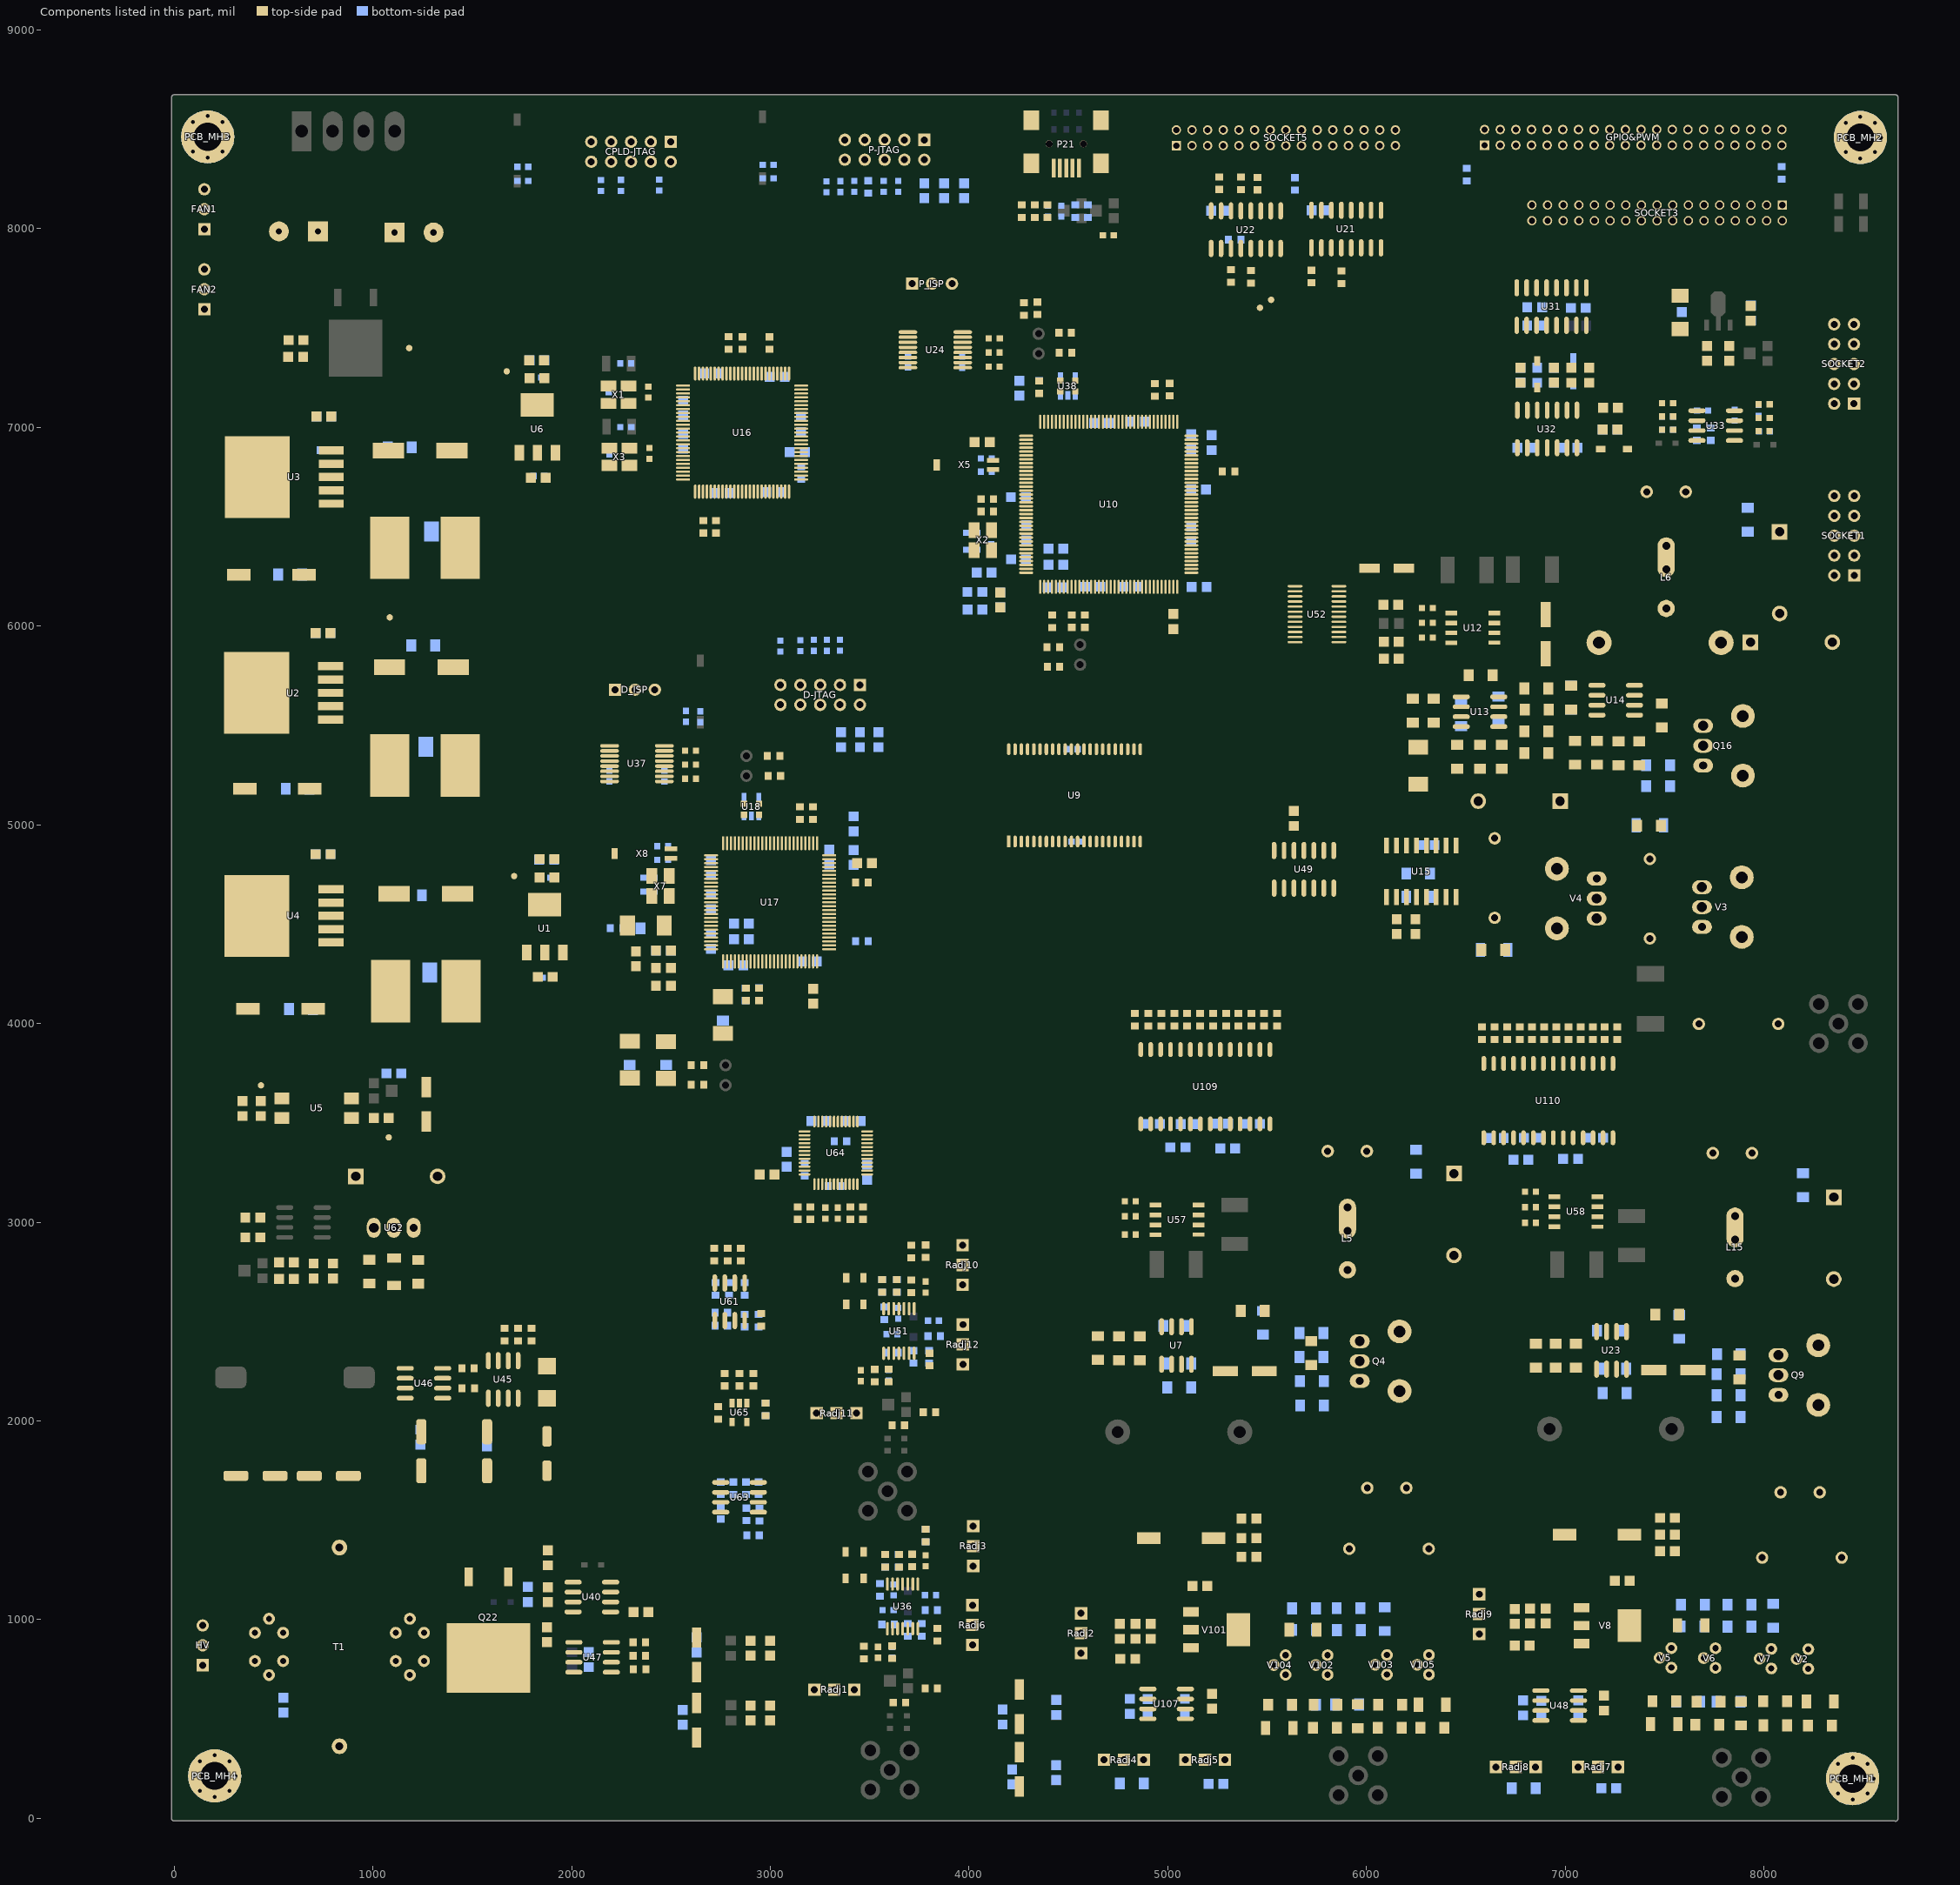
[diagram p0: the components of this part, seen from the top]
# Altium PCB MISC82309.PcbDoc (part 3 of 14)
Units mil, origin at the board's own origin, x right, y up, seen from the top; angles counter-clockwise.
Board outline 8687.03 x 8687.86 mil, 4 copper layers (Top Layer, GND, POWER, Bottom Layer); 747 components, 583 nets, 2530 pads, 1834 vias.

## Components (designator, comment, footprint, x,y, rotation, side; value= is the part's Value field where it differs from the comment) (continued)
R187 "200K" RES_0603 3470,835 r90 top
R188 "6.8K" RES_0603 3593,975 r0 bottom
R189 "6.8K" RES_0603 3646,1297 r90 bottom
R190 "18K" RES_0603 3577,1297 r270 bottom
R191 "27K" RES_0603 3577,1297 r90 top
R192 "15K" RES_0603 3552,1150 r90 bottom
R193 "3.9K" RES_0603 3647,1297 r90 top
R194 "1.5K" RES_0603 3713,1298 r270 top
R195 "27K" RES_0603 3782,1424 r270 bottom
R196 "30K" RES_0603 3782,1424 r270 top
R197 "15K" RES_0603 3761,948 r90 bottom
R198 "1K" RES_0603 3691,948 r270 bottom
R199 "100K" RES_0603 3841,924 r90 top
R200 "10K" RES_0603 3810,1048 r0 bottom
R201 "390R" R1206 5565,572 r180 top
R202 "2K2" R1206 5956,514 r270 top
R203 "100R" R1206 5791,456 r0 top
R204 "100R" R0805 3000,530 r90 top
R205 "100R" R0805 2999,856 r90 top
R206 "1K" R1206 2406,4479 r0 bottom
R207 "1K" R1206 2292,3851 r90 bottom
R208 "4.7K" R0603 4535,7208 r270 top
R209 "4.7K" R0603 4459,7208 r270 top
R212 "100R" R0805 6797,6898 r0 bottom
R213 "33R" RES_0603 1480,2165 r0 top
R214 "33R" RES_0603 1479,2265 r0 top
R215 "33R" RES_0805 1877,924 r270 top
R216 "150K" R0805 1881,1126 r270 top
R217 "100K" R0805 1880,1311 r90 top
R220 "1K" R0805 2349,1039 r0 top
R221 "1K8" R1206 6852,2329 r90 top
R222 "0R" R0805 2324,4326 r270 top
R225 "47R" R0805 2702,4414 r90 bottom
R226 "1K" RES_0603 4599,8088 r90 bottom
R227 "150K" R1206 7514,2535 r0 top
R232 "10K" R0603 2248,8218 r270 bottom
R234 "10K" R0603 2148,8217 r270 bottom
R235 "0R" R0805 2462,4190 r180 top
R236 "56K" R1206 7573,2474 r270 bottom
R269 "0R" R0805 4076,6268.51 r180 bottom
R270 "1K" RES_0603 4425,5795 r180 top
R271 "1K" RES_0603 4484,7476 r0 top
R272 "1K" RES_0603 2634,3691 r180 top
R273 "1K" RES_0603 3017,5347 r0 top
R274 "0R" RES_0603 4353,7202.5 r90 top
R275 "0R/NC" RES_0603 4353,7203 r270 bottom
R276 "47R" R0805 4249,6336 r0 bottom
R277 "0R" R0805 4030,6083 r180 bottom
R283 "4.7K" R0805 7713,7373 r270 top
R284 "560R" R0805 7825,7372 r90 top
R285 "100R" RES_0603 1731,2435 r270 top
R286 "10K" RES_0603 1799,2435 r90 top
R287 "10K" RES_0603 2342,751 r0 top
R288 "100R" RES_0603 2341,818 r180 top
R290 "50R" RES_0805 7066,556 r90 bottom
R291 "470R" RES_0805 7287,1195 r0 top
R292 "3K3" RES_0805 7194,580 r270 top
R293 "0R" RES_0805 550,570 r270 bottom
R294 "10K" R0603 2441,8219 r90 bottom
R295 "2K7" RES_0805 7514,1427 r0 top
R296 "2K7" RES_0805 7514,1512 r180 top
R297 "1K" R1206 8046,1019 r90 bottom
R298 "1K5" R1206 7721,588 r0 top
R299 "1K5" R1206 8056,589 r0 top
R300 "390R" R1206 7499,589 r180 top
R301 "390R" R1206 8282,467 r0 top
R302 "2K2" R1206 7884,528 r270 top
R303 "100R" R1206 7714,472 r0 top
R304 "100R" R1206 8057,468 r0 top
R305 "150K" R1206 7618,588 r180 bottom
R306 "1.8K" R1206 7822,588 r180 bottom
R307 "12K" R1206 7876,965 r180 bottom
R308 "12K" R1206 7876,1075 r0 bottom
R309 "12K" R1206 7643,1075 r0 bottom
R310 "12K" R1206 7640,966 r180 bottom
R312 "10K" R0603 4811.5,3030 r180 top
R313 "1M" R1206 8196,3186 r270 bottom
R314 "50R" RES_0805 6746,1017 r270 top
R315 "510R" RES_0805 6788,556 r90 bottom
R316 "50R" RES_0805 6901,1018 r90 top
R317 "20R" RES_0805 6823,1018 r270 top
R318 "2K" RES_0805 6777,3315 r0 bottom
R319 "1M" R1206 6952,2329 r90 top
R320 "2.7K" RES_0805 6879,555 r270 bottom
R321 "100R" RES_0805 6784,869 r0 top
R322 "10K" RES_0603 3595,2229 r90 top
R323 "200K" RES_0603 3526,2228 r90 top
R324 "6.8K" RES_0603 3611,2343 r0 bottom
R325 "6.8K" RES_0603 3637,2680 r90 bottom
R326 "18K" RES_0603 3563,2680 r270 bottom
R327 "27K" RES_0603 3563,2680 r90 top
R328 "15K" RES_0603 3574,2542 r90 bottom
R329 "3.9K" RES_0603 3636,2680 r90 top
R330 "1.5K" RES_0603 3709,2677 r270 top
R331 "27K" RES_0603 3710,2853 r270 top
R332 "30K" RES_0603 3782,2854 r270 top
R333 "15K" RES_0603 3721,2322 r90 bottom
R334 "1K" RES_0603 3800,2322 r270 bottom
R336 "10K" RES_0603 3825,2428 r0 bottom
R339 "100K" RES_0603 3802,2309 r90 top
R343 "10K" R0603 6825,2997 r180 top
R344 "10K" R0603 6825,3076 r180 top
R345 "0R" RES_0603 2663,6500 r270 top
R346 "0R" RES_0603 2727,6500 r270 top
R347 "0R" RES_0603 2996,7424 r90 top
R348 "0R/NC" RES_0603 4583,6025 r270 top
R349 "0R/NC" RES_0603 4517,6025 r270 top
R358 "0R" RES_0603 6504,8272 r270 bottom
R372 "330K" R0603 8001,7116 r0 top
R373 "1M" R0603 8001,7048 r0 top
R374 "330K" R0603 7973,7085 r90 bottom
R375 "0ohm" R0603 8000,6982 r180 top
R378 "4.7K" RES_0603 3810,655 r0 top
R379 "4.7K" RES_0603 3801,2045 r0 top
R386 "100R" R0805 5635,5032 r90 top
R391 "0R/NC" RES_0603 4092,6577 r180 top
R392 "0R" RES_0603 4092,6639.17 r180 top
R399 "100R" RES_0805 396,2924 r180 top
R404 "10K" RES_0603 8090,8281 r90 bottom
R405 "0R" RES_0603 5318,7762 r90 top
R406 "0R" RES_0603 3492,8210 r90 bottom
R407 "0R" RES_0603 5724,7759 r90 top
R408 "0R" RES_0603 5418,7758 r90 top
R409 "0R/NC" RES_0603 2861,7424 r90 top
R410 "0R/NC" RES_0603 2790,7425 r90 top
R411 "51R" RES_0603 2942,2505 r90 bottom
R412 "499R" RES_0603 2871,2505.51 r270 bottom
R413 "499R" RES_0603 2792,2664 r270 bottom
R414 "499R" RES_0603 2753,2480 r0 bottom
R415 "33R" RES_0603 3202,3046 r90 top
R416 "33R" RES_0603 3137,3046 r270 top
R417 "499R" RES_0603 2872,2664 r270 bottom
R418 "33R" RES_0603 3403,3046 r270 top
R419 "33R" RES_0603 3466,3046 r90 top
R455 "0R/NC" RES_0603 3156,6770 r270 bottom
R478 "0R/NC" RES_0603 2954,2509 r270 top
R479 "0R" RES_0603 2770,2208 r90 top
R491 "680R" R0805 7120,7262 r270 top
R493 "680R" R0805 7228,7098 r180 top
R495 "1K" R0805 6944,7262 r270 bottom
R496 "1K" R0805 7225,6989 r180 top
R508 "0R" RES_0603 5306,6778 r0 top
R509 "0R" RES_0603 5009,7190 r270 top
R511 "0R" RES_0603 4936,7188 r270 top
R513 "0R" RES_0603 3214,5059 r90 top
R514 "0R" RES_0603 3150,5059 r90 top
R515 "0R/NC" RES_0603 2877,4147 r270 top
R516 "0R/NC" RES_0603 2943,4147 r270 top
R517 "499R" RES_0603 2750,1538 r270 bottom
R518 "0R" RES_0603 3461,4709 r0 top
R519 "0R" RES_0603 3461,4414 r0 bottom
R521 "51R" RES_0603 2913,1425 r180 bottom
R522 "499R" RES_0603 2879,1530 r270 bottom
R523 "499R" RES_0603 2942,1661 r270 bottom
R524 "499R" RES_0603 2750.51,1661 r270 bottom
R525 "0R" RES_0603 5098,4019 r90 top
R526 "0R" RES_0603 5163,4019 r90 top
R527 "0R" RES_0603 5228,4019 r90 top
R528 "0R" RES_0603 5293,4019 r90 top
R529 "0R" RES_0603 5356,4019 r90 top
R530 "0R" RES_0603 5421,4019 r90 top
R531 "0R" RES_0603 5485,4019 r90 top
R532 "0R" RES_0603 5550,4019 r90 top
R533 "0R" RES_0603 6581,3951.5 r90 top
R534 "0R" RES_0603 6645,3951.5 r90 top
R535 "0R" RES_0603 6708,3951.5 r90 top
R536 "0R" RES_0603 6771,3951.5 r90 top
R537 "0R" RES_0603 6832,3951.5 r90 top
R538 "0R" RES_0603 6893,3951.5 r90 top
R539 "0R" RES_0603 6955,3951.5 r90 top
R540 "0R" RES_0603 7016,3951.5 r90 top
R541 "0R" RES_0603 7077,3951.5 r90 top
R542 "0R" RES_0603 7138,3951.5 r90 top
R543 "0R" RES_0603 7199,3951.5 r90 top
R544 "0R" RES_0603 7262,3951.5 r90 top
R545 "1M/NC" RES_0603 3650,583 r180 top
R546 "1M/NC" RES_0603 3644,1978 r180 top
R547 "0R" RES_0603 4835,4019 r90 top
R548 "0R" RES_0603 4902,4019 r90 top
R549 "0R" RES_0603 4968,4019 r90 top
R550 "0R" RES_0603 5034,4019 r90 top
R555 "0R/NC" RES_0603 767,6885 r0 bottom
R556 "0R" RES_0603 2227,4479 r180 bottom
R558 "0R" RES_0603 4418,6024 r270 top
R564 "0R/NC" RES_0603 2943,4148 r90 bottom
R565 "0R/NC" RES_0603 2876,4147 r90 bottom
R567 "0R/NC" RES_0603 4343,7599 r270 top
R569 "0R/NC" RES_0603 4276,7596 r270 top
R578 "0R/NC" RES_0603 2945,1529 r270 bottom
R587 "10K" R0603 3570,8213 r270 bottom
R588 "10K" R0603 3353,8212 r270 bottom
R589 "10K" R0603 3643,8213 r270 bottom
R590 "10K" R0603 3423,8213 r270 bottom
R591 "10K" R0603 3283,8211 r90 bottom
R592 "10K" R0603 3351,5904 r90 bottom
R593 "10K" R0603 3219,5903 r90 bottom
R594 "10K" R0603 3151,5902 r90 bottom
R595 "10K" R0603 3051,5899 r270 bottom
R596 "10K" R0603 3285,5903 r270 bottom
R598 "10K" RES_0603 2852,2838 r90 top
R599 "10K" RES_0603 2785,2838 r270 top
Radj1 "10K" Radj 3422,648 r180 top
Radj2 "10K" Radj 4564,832 r90 top
Radj3 "10K" Radj 4021,1470 r270 top
Radj4 "2K" Radj 4679,295 r0 top
Radj5 "5K" Radj 5088,295 r0 top
Radj6 "10K" Radj 4017,1073 r270 top
Radj7 "5K" Radj 7065,259 r0 top
Radj8 "2K" Radj 6651,259 r0 top
Radj9 "10K" Radj 6567,928 r90 top
Radj10 "10K" Radj 3967,2885 r270 top
Radj11 "10K" Radj 3433,2039 r180 top
Radj12 "10K" Radj 3969,2485 r270 top
SOCKET1 "IDC2X5-2_54" IDC2X5-2_54 8454,6255 r90 top
SOCKET2 "IDC2X5-2_54" IDC2X5-2_54 8453,7119 r90 top
SOCKET3 "HEAD2X17-2MM-A" IDC2X17-2.0mm-A 8092,8119 r180 top
SOCKET5 "HEAD2X15-2MM-A" IDC2X15-2.0mm-A 5043,8418 r0 top
T1 "Trans1" RM8 832,863 r180 top
TC2 "220uF/25V" E8X10,2 4904,1411 r0 top
TC3 "220uF/25V" E8X10,2 6997,1427 r0 top
TP1 "TP" TPOINT 1711,4742 r90 top
TP2 "TP" TPOINT 1085,6044 r90 top
TP3 "TP" TPOINT 1080,3427 r270 top
TP4 "TP" TPOINT 437,3689 r270 top
TP5 "TP" TPOINT 1183,7399 r90 top
TP6 "TP" TPOINT 1674,7282 r90 top
TP7 "TP" TPOINT 5520,7642 r90 top
TP8 "TP" TPOINT 5464,7602 r90 top
U1 "AMS1117-3.3V" SOT223 1775,4358 r90 top
U2 "LM2596S-12" TS5B_N 551,5664 r180 top
U3 "LM2596S-5.0" TS5B_N 554,6750 r180 top
U4 "LM2596S-12" TS5B_N 553,4542 r180 top
U5 "PC817" SOIC_4N 718,3574 r180 top
U6 "AMS1117-3.3V" SOT223 1738,6872 r90 top
U7 "UC3842D" SOIC-8 5044,2380 r270 top
U9 "IS61LV51216AL" TSOP44-IS61LV51216AL-10TLI 4200,4916 r90 top
U10 "STM32F407ZET6" LQFP144 4703,6613 r0 top
U12 "ISP742RI" P-DSO-8 6427,6066 r0 top
U13 "TL082ACD" SO8 6571,5569 r0 top
U14 "UC3842D" SOIC-8 7254,5627 r0 top
U15 "IR2113" SOIC-16 6276,4766 r90 top
U16 "EPM240GT100C5N" TQFP100_N 2858,6974 r270 top
U17 "STM32F407VGT6" LQFP100_N 2999,4610 r0 top
U18 "DS28CM00R-A00+T" U5+1_N 2905,5092 r90 bottom
U21 "MC3487D" 751B-03_N 5898,7998 r90 top
U22 "MC3486D" 751B-03_N 5393,7995 r90 top
U23 "UC3842D" SOIC-8 7233,2355 r270 top
U24 "SP3232EEA" SSOP16_M 3830,7390 r180 top
U31 "MC3486D" 751B-03 6931,7608 r270 top
U32 "M74HCT14M1R" SO14_N 6909,6992 r270 top
U33 "LM358D" SO8_N 7757,7009 r180 top
U36 "MC33074DTB" 948G-01_N 3666,1067 r90 top
U37 "SP3232EEA" SSOP16_M 2329,5308 r180 top
U38 "DS28CM00R-A00+T" U5+1_N 4497,7208 r90 bottom
U40 "LM358D" SO8_N 2102,1114 r0 top
U45 "IR2184S" SOIC_8N 1656,2209 r270 top
U46 "IRF7341" SOIC_8N 1257,2190 r180 top
U47 "MC33152D" 751-05_N 2106,811 r180 top
U48 "TLE2082AID" SOIC-8 6972,568 r180 top
U49 "M74HCT14M1R" SO14 5685,4776 r90 top
U51 "MC33074DTB" 948G-01_N 3647,2453 r90 top
U52 "SN74LVC4245PW" TSSOP-24 5751,6060 r180 top
U57 "ISP742RI" P-DSO-8 4939,3087 r0 top
U58 "ISP742RI" P-DSO-8 6946,3128 r0 top
U61 "ADC8138" SO8 2796,2600 r270 top
U62 "MC7815ACT" TO220 1105,2972 r90 top
U63 "ADC8138" SO8_N 2845,1616 r180 top
U64 "AD9288BST100" LQFP48A 3330,3349 r90 top
U65 "TPS60403" SOT23-5_M 2845,2042 r90 top
U107 "TLE2082AID" SOIC-8 4994,576 r180 top
U109 "DAC902" SOP127P1020X265-28N 5189,3682 r270 top
U110 "DAC902" SOP127P1020X265-28N 6915,3612 r270 top
V1 "3V3" DO-213AA 1107,2751 r90 top
V2 "TP2535N3" TO-92 8223,802 r0 top
V3 "IRF740" TO220V1 7688,4586 r0 top
V4 "IRF740" TO220V1 7158,4629 r180 top
V5 "VN0640N3" TO-92 7534,808 r0 top
V6 "BF393" TO-92 7756,807 r0 top
V7 "BF493" TO-92 8037,804 r0 top
V8 "BF720" SOT223 7083,1060 r0 top
V10 "3V3" SOD-123 3379,1275 r270 top
V11 "3V3" SOD-123 3470,1275 r270 top
V12 "3V3" SOD-123 3469,2654 r270 top
V13 "3V3" SOD-123 3382,2654 r270 top
V101 "BF720" SOT223 5116,1039 r0 top
V102 "BF393" TO-92 5804,772 r0 top
V103 "BF493" TO-92 6103,773 r0 top
V104 "VN0640N3" TO-92 5593,772 r0 top
V105 "TP2535N3" TO-92 6314,773 r0 top
X1 "24M" SMD5032 2187,7121 r0 top
X2 "8M" SMD5032 4026,6483 r270 top
X3 "16.368M" SMD5032 2191,6809 r0 top
X5 "32.768KHz" Y_XTAL_T7 4131,6786 r90 top
X7 "8M" SMD5032 2404,4742 r270 top
X8 "32.768KHz" Y_XTAL_T7 2510,4830 r90 top

## Footprints (in the part's own frame and the unit in brackets; to place one, negate y for a bottom-side part, rotate by r counter-clockwise, add the part's x,y. Pads: shape width x height; smd on the part's side, far side on the other; paste and mask are expansions set on the pad)
751-05_N [mm] "SOIC, 8-Leads, Body 4.9x3.9mm, Pitch 1.27mm, IPC Medium Density"
  oval 2.2x0.6 smd: 1(-2.4,1.905) 2(-2.4,0.635) 3(-2.4,-0.635) 4(-2.4,-1.905) 5(2.4,-1.905) 6(2.4,-0.635) 7(2.4,0.635) 8(2.4,1.905)
  silkscreen extent -2.53,-2.5 0.9,2.88, body extent -1.95,-2.45 1.95,2.45, height 1.75
751B-03 [mm] "SOIC, 16-Leads, Body 9.9x3.9mm, Pitch 1.27mm, IPC Medium Density"
  oval 2.2x0.6 smd: 1(-2.4,4.445) 2(-2.4,3.175) 3(-2.4,1.905) 4(-2.4,0.635) 5(-2.4,-0.635) 6(-2.4,-1.905) 7(-2.4,-3.175) 8(-2.4,-4.445) 9(2.4,-4.445) 10(2.4,-3.175) 11(2.4,-1.905) 12(2.4,-0.635) 13(2.4,0.635) 14(2.4,1.905) 15(2.4,3.175) 16(2.4,4.445)
  silkscreen extent -2.52,-5 0.9,5.42, body extent -3.07,-4.98 3.07,4.99, height 1.78
751B-03_N [mm] "SOIC, 16-Leads, Body 9.9x3.9mm, Pitch 1.27mm, IPC Medium Density"
  oval 2.2x0.6 smd: 1(-2.4,4.445) 2(-2.4,3.175) 3(-2.4,1.905) 4(-2.4,0.635) 5(-2.4,-0.635) 6(-2.4,-1.905) 7(-2.4,-3.175) 8(-2.4,-4.445) 9(2.4,-4.445) 10(2.4,-3.175) 11(2.4,-1.905) 12(2.4,-0.635) 13(2.4,0.635) 14(2.4,1.905) 15(2.4,3.175) 16(2.4,4.445)
  silkscreen extent -2.52,-5 0.9,5.42, body extent -1.95,-4.95 1.95,4.95, height 1.75
948G-01_N [mm] "TSOP, 14-Leads, Body 5x4.4mm, Pitch 0.65mm, IPC Medium Density"
  oval 1.7x0.35 smd: 1(-2.85,1.95) 2(-2.85,1.3) 3(-2.85,0.65) 4(-2.85,0) 5(-2.85,-0.65) 6(-2.85,-1.3) 7(-2.85,-1.95) 8(2.85,-1.95) 9(2.85,-1.3) 10(2.85,-0.65) 11(2.85,0) 12(2.85,0.65) 13(2.85,1.3) 14(2.85,1.95)
  silkscreen extent -2.97,-2.55 1.6,2.8, body extent -2.25,-2.55 2.25,2.55, height 1.2
C0603 [mm]
  rect 0.8x0.8 smd: 1(-0.698,0) 2(0.698,0)
  silkscreen extent -1.42,-0.71 1.42,0.71, body extent -0.8,-0.4 0.8,0.4, height 0.4
C0805 [mil]
  rect 50x50 smd: 1(-37.5,0) 2(37.5,0)
  silkscreen extent -77,-40 77,40, body extent -42,-25 42,25, height 59
C1206 [mil] "Chip Capacitor;Body 3.2x1.6mm(LxWtyp)"
  rect 50x60 smd: 1(-60,0) 2(60,0)
  silkscreen extent -96,-42 96,40, body extent -63,-31 63,32, height 32
c1206 [mil] "Chip Capacitor;Body 3.2x1.6mm(LxWtyp)"
  rect 50x60 smd: 1(-60,0) 2(60,0)
  silkscreen extent -96,-42 96,40, body extent -63,-31 63,32, height 32
CAP-ALU-5X5_4 [mm] "ALUMINUM ELECTROLYTIC CAPACITORS 5X5.4"
  rrect50% 2.6x1.2 smd: 1(-2.2,0) 2(2.2,0)
  silkscreen extent -2.67,-2.67 2.67,2.63, body extent -2.95,-2.65 2.95,2.65, height 5.41
CAP-ALU-6_3X5_4 [mm] "ALUMINUM ELECTROLYTIC CAPACITORS 6.3X5.4"
  rrect50% 3.2x1.3 smd: 1(5,0) 2(0,0)
  silkscreen extent -0.8,-3.3 5.8,3.3, body extent -0.99,-3.3 6.01,3.3, height 5.4
CAP-EL-10X13_5-5 [mm] "Polar capacitor 10mmx13.5mm pitch 5mm"
  round 1.6 hole 0.9: 1(2.5,0) 2(-2.5,0)
  silkscreen extent -5,-5 5,5, body extent -5,-4.99 5,4.99, height 14
CAP-EL-12x20 [mm]
  rect 2.54x2.54 hole 0.8: 1(-2.5,0)
  round 2.54 hole 0.8: 2(2.5,0)
  silkscreen extent -6.4,-6.4 6.4,6.4, body extent -6.25,-6.23 6.25,6.23, height 20.5
CAP_0603 [mm]
  rect 0.9x1 smd: 1(-0.8,0) 2(0.8,0)
  silkscreen extent -1.45,-0.7 1.45,0.7, body extent -0.8,-0.4 0.8,0.41, height 0.4
CAP_0805 [mil]
  rect 50x50 smd: 1(-37.5,0) 2(37.5,0)
  silkscreen extent -70,-32 70,32, body extent -40,-25 40,25, height 24
CAP_AVX-A [mil]
  rect 50x60 smd: 1(-60,0) 2(60,0)
  silkscreen extent -96,-47 97,47, body extent -67,-33 67,33, height 67
CBB-400V-10mm [mil] "CBB capacitor 400V"
  round 62 hole 35: 1(-200,0) 2(200,0)
  silkscreen extent -270,-100 270,100, body extent -226,-108 226,108, height 453
D2PAK_N [mm] "D2-PAK, 4-Leads, Body 8.8x10.4mm, Pitch 2.54mm, Lead Span 15.1mm, IPC Medium Density"
  rect 2.4x1.05 smd: 1(-6.8,2.54) 3(-6.8,-2.54)
  rect 8.9x10.65 smd: 2(3.55,0)
  silkscreen extent -6.92,-5.25 -1.3,5.25, body extent -2.7,-5.28 6.3,5.28, height 4.69
D1810 [mil]
  rect 75x100 smd: 1(0,0) 2(185,0)
  silkscreen extent -60,-65 250,65
"DO-41 - 10.46mm" [mm] "Diode, Axial; Body 5.2 x 2.7 mm (LxDia. max), Lead Dia. 0.86 mm (max)"
  round 2 hole 1.2: 1(-5.23,0)
  rect 2x2 hole 1.2: 2(5.23,0)
  silkscreen extent -2.65,-1.4 2.75,1.4, body extent -5.66,-1.39 5.66,1.34, height 3.16
DO-201AD [mm] "Diode, Axial; Body 9.5 x 5.6 mm (LxDia. max), Lead Dia. 1.32 mm (max) pitch 15.6mm"
  round 3.2 hole 1.524: 1(0,0) 2(15.6,0)
  silkscreen extent 2.54,-2.54 12.95,2.54, body extent -0.7,-2.79 16.2,2.85, height 5.82
DO-213AA [mm] "LL-34  MINIMELF   DO-213AA"
  rect 1.2x1.8 smd: 1(-1.75,0) 2(1.75,0)
  silkscreen extent -0.94,-0.79 0.94,0.79, body extent -1.75,-0.72 1.75,0.73, height 1.43
DO-214AA [mm]
  rect 1.8x2.2 smd: 1(-2.13,0) 2(2.13,0)
  silkscreen extent -3.32,-1.51 3.32,1.51, body extent -2.65,-1.85 2.65,1.85, height 2.2
DO-214AA-L [mm] "Molded Inductor, 2-Leads, Body 4.38x3.62mm, IPC Medium Density"
  rect 2.15x2.3 smd: 1(-2.06,0) 2(2.06,0)
  silkscreen extent -2.35,-2 2.35,2, body extent -2.65,-1.88 2.65,1.82, height 2.2
DO-214AC [mil]
  rect 75x100 smd: 1(0,0) 2(185,0)
  silkscreen extent -60,-65 250,65, body extent -12,-55 204,55, height 102
E5X5.4 [mm]
  rect 2.6x1.2 smd: 1(0,0) 2(4.4,0)
  silkscreen extent -0.47,-2.63 4.83,2.67
E6.3X5.4 [mm]
  rect 3.2x1.3 smd: 1(0,0) 2(5,0)
  silkscreen extent -0.8,-3.3 5.8,3.3, body extent -0.96,-3.3 6.04,3.3, height 5.4
E8X10,2 [mm]
  rect 3x1.5 smd: 1(0,0) 2(8.3,0)
  silkscreen extent 0,-4.15 8.3,4.15, body extent -0.76,-4.15 9.14,4.15, height 10.2
E10X10.2 [mm]
  rect 4x2 smd: 1(0,0) 2(8.128,0)
  silkscreen extent -1.02,-5.08 9.14,5.08
IDC2X5-2_54 [mil]
  rect 62x62 hole 35: 1(0,0)
  round 62 hole 35: 2(0,100) 3(100,0) 4(100,100) 5(200,0) 6(200,100) 7(300,0) 8(300,100) 9(400,0) 10(400,100)
  silkscreen extent -201,-155 601,225, body extent -201,-129 601,237, height 360
IDC2X15-2.0mm-A [mm]
  rect 1.2x1.2 hole 0.8: 1(0,0)
  round 1.2 hole 0.8: 2(0,2) 3(2,0) 4(2,2) 5(4,0) 6(4,2) 7(6,0) 8(6,2) 9(8,0) 10(8,2) 11(10,0) 12(10,2) 13(12,0) 14(12,2) 15(14,0) 16(14,2) 17(16,0) 18(16,2) 19(18,0) 20(18,2) 21(20,0) 22(20,2) 23(22,0) 24(22,2) 25(24,0) 26(24,2) 27(26,0) 28(26,2) 29(28,0) 30(28,2)
  silkscreen extent -4.5,-2.6 32.5,3.75, body extent -4.5,-1.85 32.5,3.75, height 5.75
IDC2X17-2.0mm-A [mm]
  rect 1.2x1.2 hole 0.8: 1(0,0)
  round 1.2 hole 0.8: 2(0,2) 3(2,0) 4(2,2) 5(4,0) 6(4,2) 7(6,0) 8(6,2) 9(8,0) 10(8,2) 11(10,0) 12(10,2) 13(12,0) 14(12,2) 15(14,0) 16(14,2) 17(16,0) 18(16,2) 19(18,0) 20(18,2) 21(20,0) 22(20,2) 23(22,0) 24(22,2) 25(24,0) 26(24,2) 27(26,0) 28(26,2) 29(28,0) 30(28,2) 31(30,0) 32(30,2) 33(32,0) 34(32,2)
  silkscreen extent -4.5,-2.6 36.5,3.75, body extent -4.5,-1.8 36.5,3.75, height 5.75
IDC2X20-2.0mm-A [mm]
  rect 1.2x1.2 hole 0.8: 1(0,0)
  round 1.2 hole 0.8: 2(0,2) 3(2,0) 4(2,2) 5(4,0) 6(4,2) 7(6,0) 8(6,2) 9(8,0) 10(8,2) 11(10,0) 12(10,2) 13(12,0) 14(12,2) 15(14,0) 16(14,2) 17(16,0) 18(16,2) 19(18,0) 20(18,2) 21(20,0) 22(20,2) 23(22,0) 24(22,2) 25(24,0) 26(24,2) 27(26,0) 28(26,2) 29(28,0) 30(28,2) 31(30,0) 32(30,2) 33(32,0) 34(32,2) 35(34,0) 36(34,2) 37(36,0) 38(36,2) 39(38,0) 40(38,2)
  silkscreen extent -4.5,-2.6 42.5,3.75, body extent -4.5,-1.85 42.5,3.75, height 5.75
KF2510-3A [mil] "2.54mm Connect, 3Pin"
  rect 62x62 hole 35: 1(-100,0)
  round 62 hole 35: 2(0,0) 3(100,0)
  silkscreen extent -150,-160 150,102, body extent -150,-126 150,102, height 453
L200/1.4A [mm] "200uH 1.4A 4.5M"
  round 2.2 hole 1: 1(4,0) 2(-4,0)
  oval 5x2.2 hole 1 copper offset 1.5,0: 3(1,0)
  silkscreen extent -2.2,-10 2.2,10, body extent -3.71,-9.67 3.66,9.68, height 19.68
L330 [mm] "330mH/1A"
  rect 5x8 smd: 1(-0.127,0) 2(8.873,0)
  silkscreen extent -1.63,-6 10.37,6
L-9x12 [mm]
  round 1.6 hole 0.85: 1(-2.5,0) 2(2.5,0)
  silkscreen extent -4.2,-4.2 4.2,4.2, body extent -4.5,-4.5 4.5,4.5, height 13
LED_0805 [mil]
  rect 50x50 smd: 1(-37.5,0) 2(37.5,0)
  silkscreen extent -92,-33 78,33, body extent -41,-27 41,27, height 35
LQFP48A [mm]
  oval 1.5x0.3 smd: 1(-4,2.75) 2(-4,2.25) 3(-4,1.75) 4(-4,1.25) 5(-4,0.75) 6(-4,0.25) 7(-4,-0.25) 8(-4,-0.75) 9(-4,-1.25) 10(-4,-1.75) 11(-4,-2.25) 12(-4,-2.75) 25(4,-2.75) 26(4,-2.25) 27(4,-1.75) 28(4,-1.25) 29(4,-0.75) 30(4,-0.25) 31(4,0.25) 32(4,0.75) 33(4,1.25) 34(4,1.75) 35(4,2.25) 36(4,2.75)
  oval 0.3x1.5 smd: 13(-2.75,-4) 14(-2.25,-4) 15(-1.75,-4) 16(-1.25,-4) 17(-0.75,-4) 18(-0.25,-4) 19(0.25,-4) 20(0.75,-4) 21(1.25,-4) 22(1.75,-4) 23(2.25,-4) 24(2.75,-4) 37(2.75,4) 38(2.25,4) 39(1.75,4) 40(1.25,4) 41(0.75,4) 42(0.25,4) 43(-0.25,4) 44(-0.75,4) 45(-1.25,4) 46(-1.75,4) 47(-2.25,4) 48(-2.75,4)
  silkscreen extent -5.46,-2.92 2.92,3.17
LQFP100_N [mm] "Thin QFP, 100-Leads, Body 14x14mm, Pitch 0.5mm, IPC Medium Density"
  oval 1.8x0.3 smd: 1(-7.55,6) 2(-7.55,5.5) 3(-7.55,5) 4(-7.55,4.5) 5(-7.55,4) 6(-7.55,3.5) 7(-7.55,3) 8(-7.55,2.5) 9(-7.55,2) 10(-7.55,1.5) 11(-7.55,1) 12(-7.55,0.5) 13(-7.55,0) 14(-7.55,-0.5) 15(-7.55,-1) 16(-7.55,-1.5) 17(-7.55,-2) 18(-7.55,-2.5) 19(-7.55,-3) 20(-7.55,-3.5) 21(-7.55,-4) 22(-7.55,-4.5) 23(-7.55,-5) 24(-7.55,-5.5) 25(-7.55,-6) 51(7.55,-6) 52(7.55,-5.5) 53(7.55,-5) 54(7.55,-4.5) 55(7.55,-4) 56(7.55,-3.5) 57(7.55,-3) 58(7.55,-2.5) 59(7.55,-2) 60(7.55,-1.5) 61(7.55,-1) 62(7.55,-0.5) 63(7.55,0) 64(7.55,0.5) 65(7.55,1) 66(7.55,1.5) 67(7.55,2) 68(7.55,2.5) 69(7.55,3) 70(7.55,3.5) 71(7.55,4) 72(7.55,4.5) 73(7.55,5) 74(7.55,5.5) 75(7.55,6)
  oval 0.3x1.8 smd: 26(-6,-7.55) 27(-5.5,-7.55) 28(-5,-7.55) 29(-4.5,-7.55) 30(-4,-7.55) 31(-3.5,-7.55) 32(-3,-7.55) 33(-2.5,-7.55) 34(-2,-7.55) 35(-1.5,-7.55) 36(-1,-7.55) 37(-0.5,-7.55) 38(0,-7.55) 39(0.5,-7.55) 40(1,-7.55) 41(1.5,-7.55) 42(2,-7.55) 43(2.5,-7.55) 44(3,-7.55) 45(3.5,-7.55) 46(4,-7.55) 47(4.5,-7.55) 48(5,-7.55) 49(5.5,-7.55) 50(6,-7.55) 76(6,7.55) 77(5.5,7.55) 78(5,7.55) 79(4.5,7.55) 80(4,7.55) 81(3.5,7.55) 82(3,7.55) 83(2.5,7.55) 84(2,7.55) 85(1.5,7.55) 86(1,7.55) 87(0.5,7.55) 88(0,7.55) 89(-0.5,7.55) 90(-1,7.55) 91(-1.5,7.55) 92(-2,7.55) 93(-2.5,7.55) 94(-3,7.55) 95(-3.5,7.55) 96(-4,7.55) 97(-4.5,7.55) 98(-5,7.55) 99(-5.5,7.55) 100(-6,7.55)
  silkscreen extent -7.67,-6.25 6.25,6.82, body extent -7,-7 7,7, height 1.6
LQFP144 [mm]
  oval 1.8x0.3 smd: 1(-10.55,8.75) 2(-10.55,8.25) 3(-10.55,7.75) 4(-10.55,7.25) 5(-10.55,6.75) 6(-10.55,6.25) 7(-10.55,5.75) 8(-10.55,5.25) 9(-10.55,4.75) 10(-10.55,4.25) 11(-10.55,3.75) 12(-10.55,3.25) 13(-10.55,2.75) 14(-10.55,2.25) 15(-10.55,1.75) 16(-10.55,1.25) 17(-10.55,0.75) 18(-10.55,0.25) 19(-10.55,-0.25) 20(-10.55,-0.75) 21(-10.55,-1.25) 22(-10.55,-1.75) 23(-10.55,-2.25) 24(-10.55,-2.75) 25(-10.55,-3.25) 26(-10.55,-3.75) 27(-10.55,-4.25) 28(-10.55,-4.75) 29(-10.55,-5.25) 30(-10.55,-5.75) 31(-10.55,-6.25) 32(-10.55,-6.75) 33(-10.55,-7.25) 34(-10.55,-7.75) 35(-10.55,-8.25) 36(-10.55,-8.75) 73(10.55,-8.75) 74(10.55,-8.25) 75(10.55,-7.75) 76(10.55,-7.25) 77(10.55,-6.75) 78(10.55,-6.25) 79(10.55,-5.75) 80(10.55,-5.25) 81(10.55,-4.75) 82(10.55,-4.25) 83(10.55,-3.75) 84(10.55,-3.25) 85(10.55,-2.75) 86(10.55,-2.25) 87(10.55,-1.75) 88(10.55,-1.25) 89(10.55,-0.75) 90(10.55,-0.25) 91(10.55,0.25) 92(10.55,0.75) 93(10.55,1.25) 94(10.55,1.75) 95(10.55,2.25) 96(10.55,2.75) 97(10.55,3.25) 98(10.55,3.75) 99(10.55,4.25) 100(10.55,4.75) 101(10.55,5.25) 102(10.55,5.75) 103(10.55,6.25) 104(10.55,6.75) 105(10.55,7.25) 106(10.55,7.75) 107(10.55,8.25) 108(10.55,8.75)
  oval 0.3x1.8 smd: 37(-8.75,-10.55) 38(-8.25,-10.55) 39(-7.75,-10.55) 40(-7.25,-10.55) 41(-6.75,-10.55) 42(-6.25,-10.55) 43(-5.75,-10.55) 44(-5.25,-10.55) 45(-4.75,-10.55) 46(-4.25,-10.55) 47(-3.75,-10.55) 48(-3.25,-10.55) 49(-2.75,-10.55) 50(-2.25,-10.55) 51(-1.75,-10.55) 52(-1.25,-10.55) 53(-0.75,-10.55) 54(-0.25,-10.55) 55(0.25,-10.55) 56(0.75,-10.55) 57(1.25,-10.55) 58(1.75,-10.55) 59(2.25,-10.55) 60(2.75,-10.55) 61(3.25,-10.55) 62(3.75,-10.55) 63(4.25,-10.55) 64(4.75,-10.55) 65(5.25,-10.55) 66(5.75,-10.55) 67(6.25,-10.55) 68(6.75,-10.55) 69(7.25,-10.55) 70(7.75,-10.55) 71(8.25,-10.55) 72(8.75,-10.55) 109(8.75,10.55) 110(8.25,10.55) 111(7.75,10.55) 112(7.25,10.55) 113(6.75,10.55) 114(6.25,10.55) 115(5.75,10.55) 116(5.25,10.55) 117(4.75,10.55) 118(4.25,10.55) 119(3.75,10.55) 120(3.25,10.55) 121(2.75,10.55) 122(2.25,10.55) 123(1.75,10.55) 124(1.25,10.55) 125(0.75,10.55) 126(0.25,10.55) 127(-0.25,10.55) 128(-0.75,10.55) 129(-1.25,10.55) 130(-1.75,10.55) 131(-2.25,10.55) 132(-2.75,10.55) 133(-3.25,10.55) 134(-3.75,10.55) 135(-4.25,10.55) 136(-4.75,10.55) 137(-5.25,10.55) 138(-5.75,10.55) 139(-6.25,10.55) 140(-6.75,10.55) 141(-7.25,10.55) 142(-7.75,10.55) 143(-8.25,10.55) 144(-8.75,10.55)
  silkscreen extent -10.67,-9.25 9.25,9.57, body extent -10,-10 10,10, height 1.6
MiniUSB-A [mm]
  rect 2.4x0.5 smd: 1(3.1,1.6) 2(3.1,0.8) 3(3.1,0) 4(3.1,-0.8) 5(3.1,-1.6)
  rect 2.5x2 smd: 6(-3,4.45) 7(2.5,4.45) 8(-3,-4.45) 9(2.5,-4.45)
  round 0.9 hole 0.9: 10(0,2.2) 11(0,-2.2)
  silkscreen extent -6,-5.72 4.57,5.72, body extent -5.89,-5.36 3.31,5.34, height 3.95
MOUNTING_HOLE_3MM [mm]
  round 4 hole 3.6: 0(0,0)
  round 0.5 hole 0.5: 1(0,2.667) 2(1.886,1.886) 3(2.667,0) 4(1.886,-1.886) 5(0,-2.667) 6(-1.886,-1.886) 7(-2.667,0) 8(-1.886,1.886)
  round 6.8 smd: 9(0,0)
  round 6.8 smd far side: 10(0,0)
  silkscreen extent -3.54,-3.54 3.54,3.54